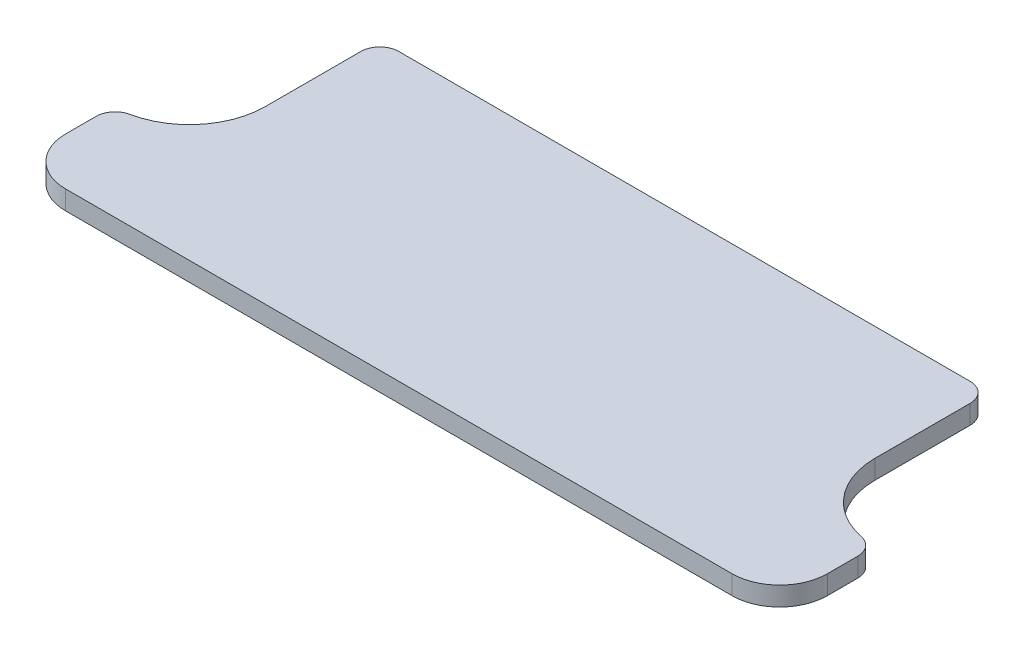
from build123d import *

# Parameters (mm, degrees)
BOSS_EXTRUDE1_DEPTH = 20
FILLET1_R           = 50
FILLET2_R           = 20


with BuildPart() as part:
    # Sketch1 → Boss-Extrude1 (new body)
    with BuildSketch(Plane(origin=(0, 0, 0), x_dir=(1, 0, 0), z_dir=(0, 1, 0))):
        with BuildLine():
            Line((-320, 150), (-320, 30))
            ThreePointArc((-320, 30), (-343.431457505, -26.568542495), (-400, -50))
            Line((-400, -50), (-400, -150))
            Line((-400, -150), (400, -150))
            Line((400, -150), (400, -50))
            ThreePointArc((400, -50), (343.431457505, -26.568542495), (320, 30))
            Line((320, 30), (320, 150))
            Line((320, 150), (-320, 150))
        make_face()
    extrude(amount=-BOSS_EXTRUDE1_DEPTH)

    # Fillet1
    fillet1_edges = [part.edges().sort_by_distance(p)[0] for p in [
        (400, -10, 150),
        (-400, -10, 150),
    ]]
    fillet(fillet1_edges, radius=FILLET1_R)

    # Fillet2
    fillet2_edges = [part.edges().sort_by_distance(p)[0] for p in [
        (-400, -10, 50),
        (-320, -10, -150),
        (320, -10, -150),
        (400, -10, 50),
    ]]
    fillet(fillet2_edges, radius=FILLET2_R)


solid = part.part
